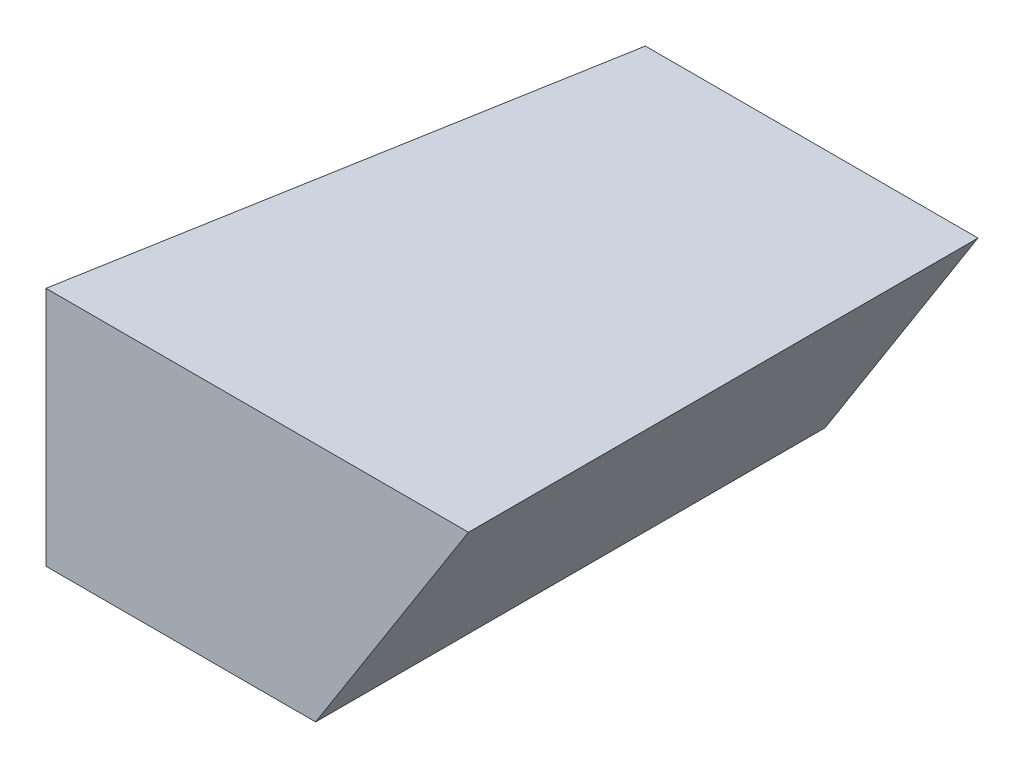
SolidWorks part; units mm, degrees
ref_plane "前视基准面" through (0, 0, 0) normal (0, 0, 1) x (1, 0, 0)
ref_plane "上视基准面" through (0, 0, 0) normal (0, 1, 0) x (1, 0, 0)
ref_plane "右视基准面" through (0, 0, 0) normal (1, 0, 0) x (0, 0, -1)
sketch "草图1" plane through (0, 0, 0) normal (0, 0, 1) x (1, 0, 0)
  line L3 (-4.4079, 5) -> (-7.4079, 5)
  line L4 (-7.4079, 5) -> (-7.4079, 6.5)
  line L6 (-7.4079, 6.5) -> (-3.4554, 6.5)
  line L13 (-3.4554, 6.5) -> (-4.4079, 5)
  dimension "D1" = 3
  dimension "D2" = 0.9525
  dimension "D3" = 1.5
extrude "凸台-拉伸1" add sketch "草图1" along normal blind 3.175 contours L4 L6 L13 L3
sketch "草图2" plane through (0, 5, 0) normal (0, -1, 0) x (1, 0, 0)
  line L0 (-7.4079, 0) -> (-5.5279, 0)
  line L1 (-4.4079, 0) -> (-7.4079, 0) construction
  line L2 (-7.4079, 0) -> (-7.4079, 3.175)
  line L3 (-7.4079, 3.175) -> (-6.0879, 3.175)
  line L4 (-4.4079, 3.175) -> (-7.4079, 3.175) construction
  line L5 (-5.5279, 0) -> (-6.0879, 3.175)
  dimension "D1" = 1.88
  dimension "D2" = 1.32
extrude "切除-拉伸1" cut sketch "草图2" against normal blind 10
